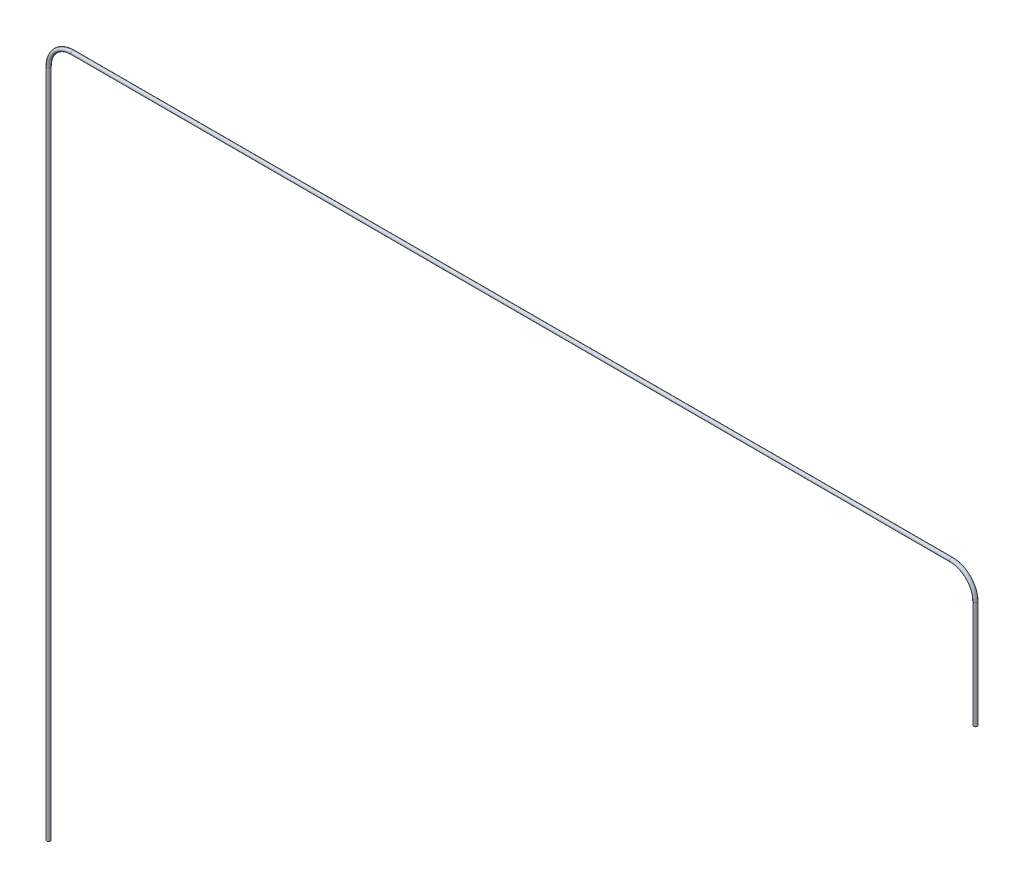
from build123d import *

# Parameters (mm, degrees)
SKETCH2_R = 3.25


with BuildPart() as part:
    # Sweep1: sweep along a path in Sketch1
    with BuildLine(Plane.XY) as sweep1_path:
        Line((0, 0), (0, 1173))
        ThreePointArc((0, 1173), (12.30151519, 1202.69848481), (42, 1215))
        Line((42, 1215), (1580, 1215))
        ThreePointArc((1580, 1215), (1609.69848481, 1202.69848481), (1622, 1173))
        Line((1622, 1173), (1622, 985))
    # Sketch2 → Sweep1 (sweep)
    with BuildSketch(Plane(origin=(0, 0, 0), x_dir=(1, 0, 0), z_dir=(0, 1, 0))):
        Circle(SKETCH2_R)
    sweep(path=sweep1_path.line)


solid = part.part
